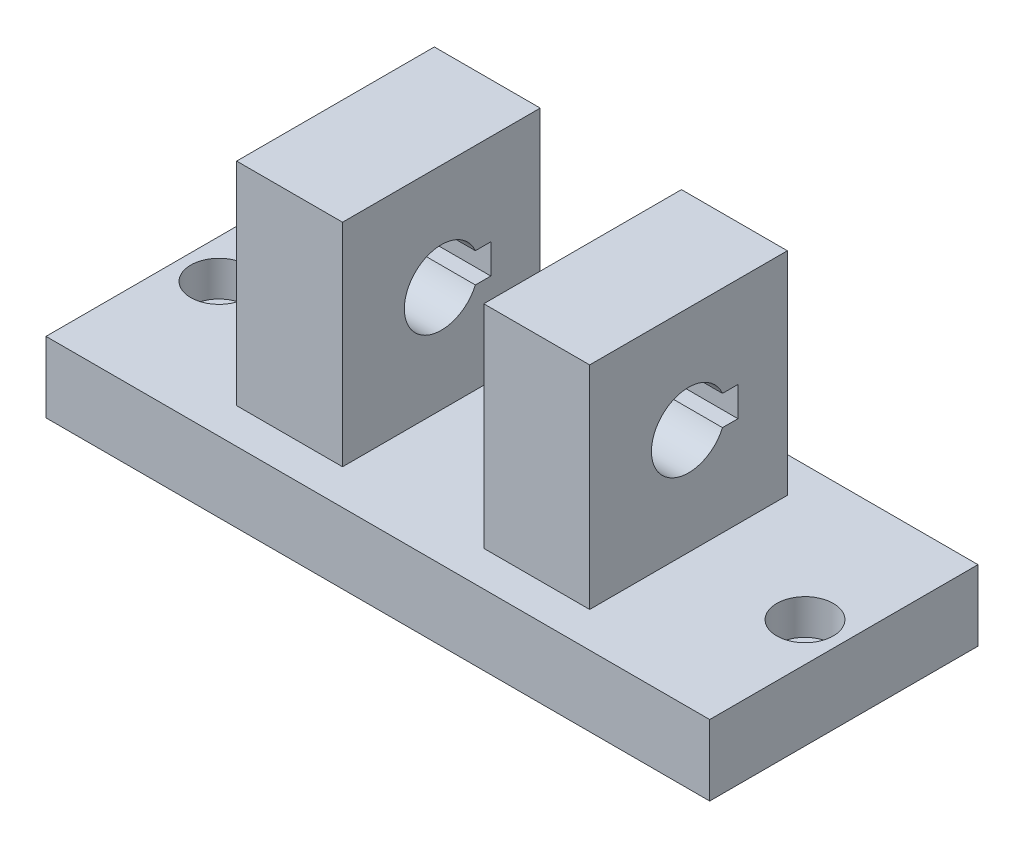
SolidWorks part; units mm, degrees
ref_plane "Front Plane" through (0, 0, 0) normal (0, 0, 1) x (1, 0, 0)
ref_plane "Top Plane" through (0, 0, 0) normal (0, 1, 0) x (1, 0, 0)
ref_plane "Right Plane" through (0, 0, 0) normal (1, 0, 0) x (0, 0, -1)
sketch "Sketch1" plane through (0, 0, 0) normal (0, 1, 0) x (1, 0, 0)
  line L1 (-47, -19) -> (47, -19)
  line L2 (-47, -19) -> (-47, 19)
  line L3 (-47, 19) -> (47, 19)
  line L4 (47, -19) -> (47, 19)
  line L5 (-47, -19) -> (47, 19) construction
  line L6 (-47, 19) -> (47, -19) construction
  point P0 (0, 0)
  dimension "D1" = 94
  dimension "D2" = 38
extrude "Boss-Extrude1" add sketch "Sketch1" along normal blind 10
sketch "Sketch2" plane through (0, 10, 0) normal (0, 1, 0) x (1, 0, 0)
  line L0 (-41.5, 0) -> (41.5, 0) construction
  circle A1 centre (-41.5, 0) radius 4
  point P4 (0, 0)
  dimension "D2" = 8
  dimension "D1" = 83
extrude "Cut-Extrude1" cut sketch "Sketch2" against normal blind 5
sketch "Sketch3" plane through (0, 5, 0) normal (0, 1, 0) x (1, 0, 0)
  circle A0 centre (-41.5, 0) radius 2.5
  dimension "D1" = 5
extrude "Cut-Extrude2" cut sketch "Sketch3" against normal blind 5
ref_plane "Plane1" through (-25, 0, 0) normal (-1, 0, 0) x (0, 0, 1)
sketch "Sketch4" plane through (-25, 0, 0) normal (-1, 0, 0) x (0, 0, 1)
  line L0 (-19, 10) -> (19, 10) construction
  line L1 (14, 10) -> (-14, 10)
  line L2 (14, 10) -> (14, 40)
  line L3 (14, 40) -> (-14, 40)
  line L4 (-14, 10) -> (-14, 40)
  line L5 (19, 10) -> (19, 0) construction
  dimension "D1" = 5
  dimension "D2" = 28
  dimension "D3" = 30
extrude "Boss-Extrude2" add sketch "Sketch4" against normal blind 15
sketch "Sketch6" plane through (-25, 0, 0) normal (-1, 0, 0) x (0, 0, 1)
  line L0 (0, 40) -> (0, 10) construction
  line L1 (14, 40) -> (-14, 40) construction
  line L2 (-19, 10) -> (19, 10) construction
  line L3 (-9.0116, 27.1) -> (16.1853, 27.1) construction
  line L4 (-8.3087, 22.9) -> (16.0101, 22.9) construction
  line L5 (-7, 27.1) -> (-4.8117, 27.1)
  line L6 (-7, 22.9) -> (-4.8117, 22.9)
  line L7 (-7, 25) -> (-7, 27.1) construction
  line L8 (-7, 27.1) -> (-7, 22.9)
  arc A0 (-4.8117, 22.9) -> (-4.8117, 27.1) centre (0, 25) ccw
  dimension "D1" = 2.1
  dimension "D2" = 2.1
extrude "Cut-Extrude3" cut sketch "Sketch6" against normal blind 109 contours L6 A0 L5 L8
mirror "Mirror1" about plane through (0, 0, 0) normal (1, 0, 0) of "Cut-Extrude2", "Cut-Extrude1", "Boss-Extrude2"
sketch "Sketch7" plane through (10, 0, 0) normal (-1, 0, 0) x (0, 0, 1)
  line L0 (-7, 22.9) -> (-4.8117, 22.9) construction
  line L1 (-7, 27.1) -> (-7, 22.9) construction
  line L2 (-7, 27.1) -> (-4.8117, 27.1) construction
  line L3 (-7, 22.9) -> (-4.8117, 22.9)
  line L4 (-7, 27.1) -> (-7, 22.9)
  line L5 (-7, 27.1) -> (-4.8117, 27.1)
  arc A0 (-4.8117, 22.9) -> (-4.8117, 27.1) centre (0, 25) ccw construction
  arc A1 (-4.8117, 22.9) -> (-4.8117, 27.1) centre (0, 25) ccw
extrude "Cut-Extrude4" cut sketch "Sketch7" against normal blind 70
